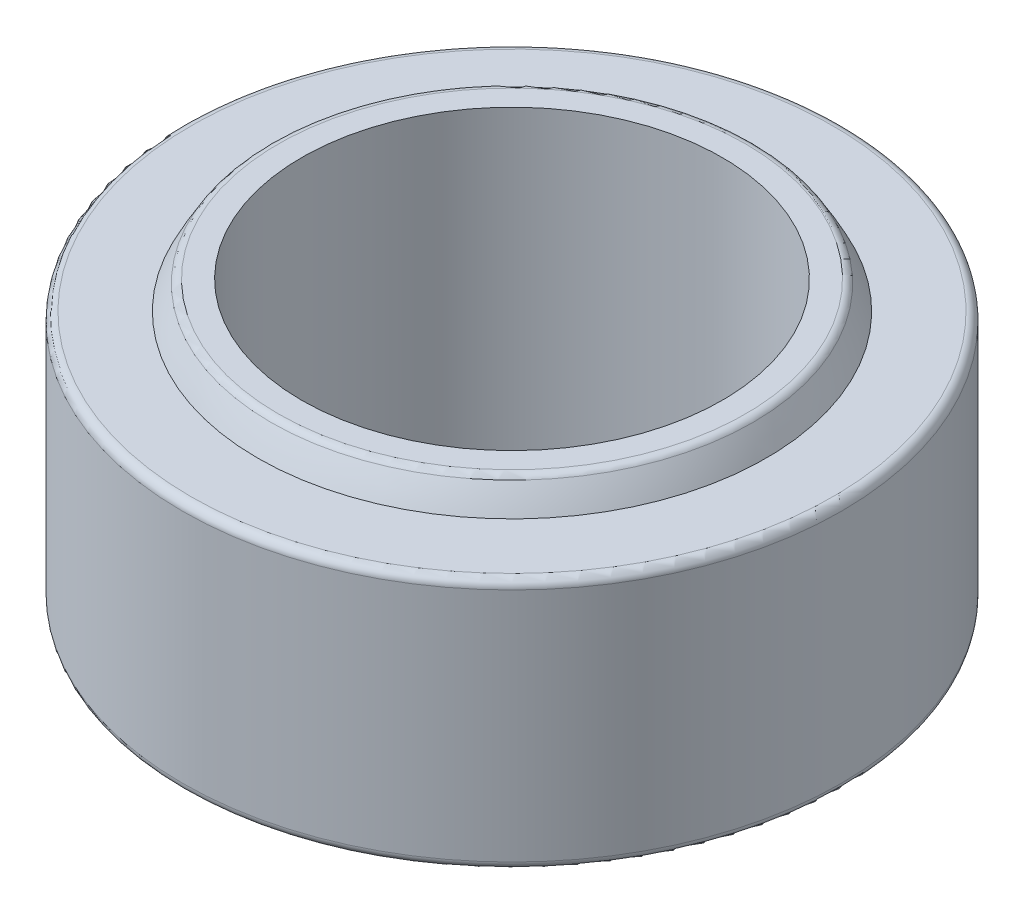
from build123d import *


with BuildPart() as part:
    # 草图2 → 旋转1 (revolve)
    with BuildSketch(Plane(origin=(0, 0, 0), x_dir=(0, 0, -1), z_dir=(1, 0, 0))):
        with BuildLine():
            Line((-22.9, 9), (-18.138357147, 9))
            ThreePointArc((-18.138357147, 9), (-20.248456731, 0), (-18.138357147, -9))
            Line((-18.138357147, -9), (-22.9, -9))
            ThreePointArc((-22.9, -9), (-23.324264069, -8.824264069), (-23.5, -8.4))
            Line((-23.5, -8.4), (-23.5, 8.4))
            ThreePointArc((-23.5, 8.4), (-23.324264069, 8.824264069), (-22.9, 9))
        make_face()
    revolve(axis=Axis((0, 11, 0), (0, -1, 0)))

    # 草图3 → 旋转2 (revolve)
    with BuildSketch(Plane(origin=(0, 0, 0), x_dir=(0, 0, -1), z_dir=(1, 0, 0))):
        with BuildLine():
            Line((-16.670388475, 11), (-15, 11))
            Line((-15, 11), (-15, -11))
            Line((-15, -11), (-16.670388475, -11))
            ThreePointArc((-16.670388475, -11), (-16.961464654, -10.924666235), (-17.179447951, -10.717582194))
            ThreePointArc((-17.179447951, -10.717582194), (-20.248456731, 0), (-17.179447951, 10.717582194))
            ThreePointArc((-17.179447951, 10.717582194), (-16.961464654, 10.924666235), (-16.670388475, 11))
        make_face()
    revolve(axis=Axis((0, 11, 0), (0, -1, 0)))


solid = part.part
